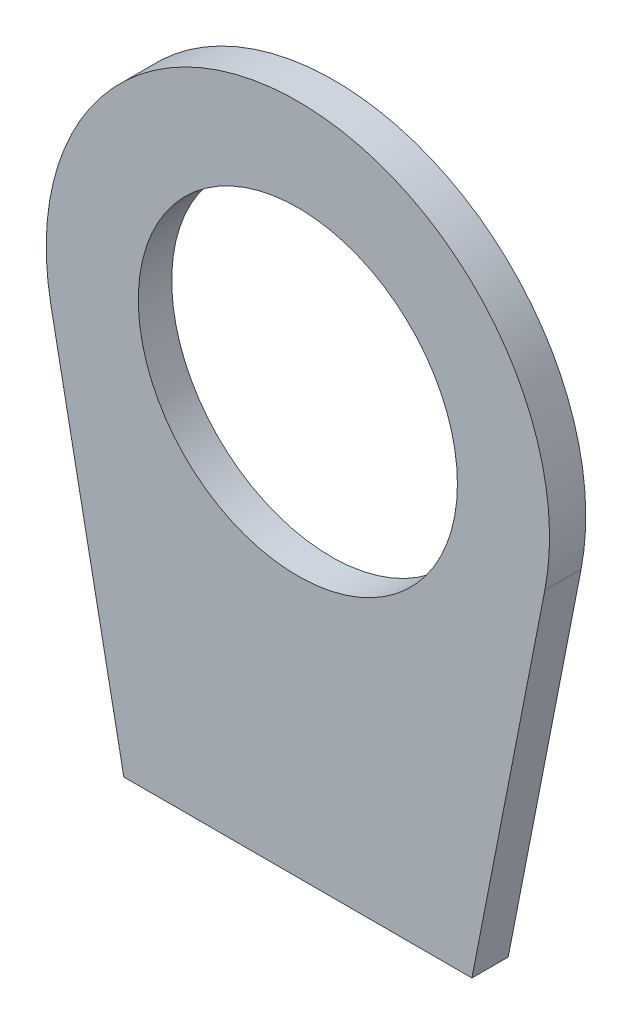
from build123d import *

# Parameters (mm, degrees)
SKETCH1_R           = 110
BOSS_EXTRUDE1_DEPTH = 25
SKETCH2_R           = 123
SKETCH2_R_2         = 110
CUT_EXTRUDE2_DEPTH  = 2


with BuildPart() as part:
    # Sketch1 → Boss-Extrude1 (new body)
    with BuildSketch(Plane.XY):
        with BuildLine():
            Line((-120, 0), (120, 0))
            Line((120, 0), (170.2653156, 256.653751283))
            ThreePointArc((170.2653156, 256.653751283), (0, 463.5), (-170.2653156, 256.653751283))
            Line((-170.2653156, 256.653751283), (-120, 0))
        make_face()
        with Locations((0, 290)):
            Circle(SKETCH1_R, mode=Mode.SUBTRACT)
    extrude(amount=BOSS_EXTRUDE1_DEPTH)

    # Sketch2 → Cut-Extrude2 (cut)
    with BuildSketch(Plane.XY):
        with Locations((0, 290)):
            Circle(SKETCH2_R)
        with Locations((0, 290)):
            Circle(SKETCH2_R_2, mode=Mode.SUBTRACT)
    extrude(amount=CUT_EXTRUDE2_DEPTH, mode=Mode.SUBTRACT)


solid = part.part
